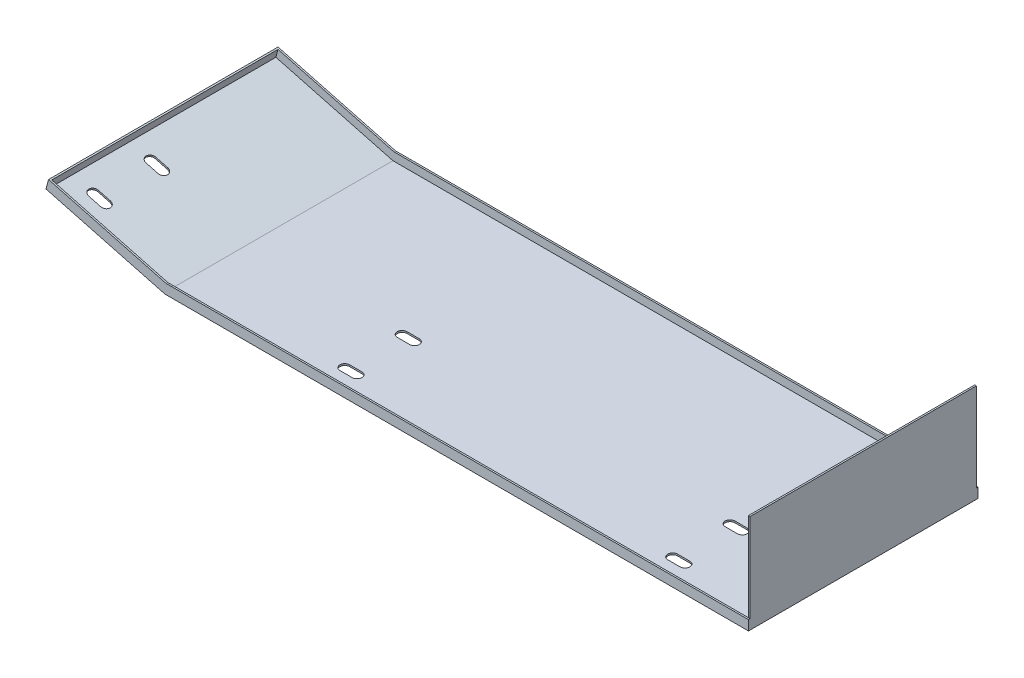
SolidWorks part; units mm, degrees
material "Plain Carbon Steel"
ref_plane "Front Plane" through (0, 0, 0) normal (0, 0, 1) x (1, 0, 0)
ref_plane "Top Plane" through (0, 0, 0) normal (0, 1, 0) x (1, 0, 0)
ref_plane "Right Plane" through (0, 0, 0) normal (1, 0, 0) x (0, 0, -1)
sketch "Sketch1" plane through (0, 0, 0) normal (0, 0, 1) x (1, 0, 0)
  line L0 (0, 0) -> (0, 120)
  line L1 (0, 0) -> (-712, 0)
  line L2 (-712, 0) -> (-856.99, 38.4434)
  dimension "D1" = 120
  dimension "D2" = 712
  dimension "D3" = 150
  dimension "D4" = 165.15
extrude "Extrude-Thin1" add sketch "Sketch1" along normal blind 276 thin thin type one direction wall 2
sketch "Sketch2" plane through (0, 0, 276) normal (0, 0, 1) x (1, 0, 0)
  line L1 (-712, 0) -> (-856.99, 38.4434)
  line L3 (0, 0) -> (-712, 0)
extrude "Extrude-Thin2" add sketch "Sketch2" along normal blind 2 thin
sketch "Sketch4" plane through (0, 0, 0) normal (0, 0, -1) x (-1, 0, 0)
  line L0 (0, 0) -> (712, 0)
  line L1 (712, 0) -> (856.99, 38.4434)
extrude "Extrude-Thin3" add sketch "Sketch4" along normal blind 2 thin thin type one direction reverse wall 12
sketch "Sketch5" plane through (0, 0, 0) normal (0, -1, 0) x (1, 0, 0)
  line L0 (-122.5, 248) -> (-107.5, 248) construction
  line L1 (-122.5, 254) -> (-107.5, 254)
  line L2 (-122.5, 242) -> (-107.5, 242)
  line L3 (0, 278) -> (-712, 278) construction
  line L4 (0, 278) -> (0, -2) construction
  arc A0 (-122.5, 254) -> (-122.5, 242) centre (-122.5, 248) ccw
  arc A1 (-107.5, 242) -> (-107.5, 254) centre (-107.5, 248) ccw
  point P2 (-115, 248)
  dimension "D1" = 6
  dimension "D2" = 15
  dimension "D3" = 30
  dimension "D4" = 115
extrude "Cut-Extrude1" cut sketch "Sketch5" against normal blind 2
pattern_linear "LPattern1" count 2 spacing 400 along (-1, 0, 0) count 2 spacing 70 along (0, 0, -1) of "Cut-Extrude1"
sketch "Sketch6" plane through (-46.7672, -176.3833, 0) normal (-0.2563, -0.9666, 0) x (0.9666, -0.2563, 0)
  line L0 (-809.7193, 248) -> (-794.7193, 248) construction
  line L1 (-809.7193, 254) -> (-794.7193, 254)
  line L2 (-809.7193, 242) -> (-794.7193, 242)
  line L3 (-688.2193, 278) -> (-838.2193, 278) construction
  line L4 (-688.2193, 278) -> (-688.2193, -2) construction
  arc A0 (-809.7193, 254) -> (-809.7193, 242) centre (-809.7193, 248) ccw
  arc A1 (-794.7193, 242) -> (-794.7193, 254) centre (-794.7193, 248) ccw
  point P2 (-802.2193, 248)
  dimension "D1" = 6
  dimension "D2" = 15
  dimension "D3" = 30
  dimension "D4" = 114
extrude "Cut-Extrude2" cut sketch "Sketch6" against normal blind 2
pattern_linear "LPattern2" count 2 spacing 70 along (0, 0, -1) of "Cut-Extrude2"
sketch "Sketch7" plane through (-46.2546, -174.4501, 0) normal (0.2563, 0.9666, 0) x (0.9666, -0.2563, 0)
  line L0 (-688.4799, -276) -> (-838.2193, -276) construction
  line L1 (-838.2193, 0) -> (-836.2193, 0)
  line L2 (-838.2193, 0) -> (-838.2193, -276)
  line L3 (-838.2193, -276) -> (-836.2193, -276)
  line L4 (-836.2193, 0) -> (-836.2193, -276)
  dimension "D1" = 2
extrude "Boss-Extrude1" add sketch "Sketch7" along normal blind 10
